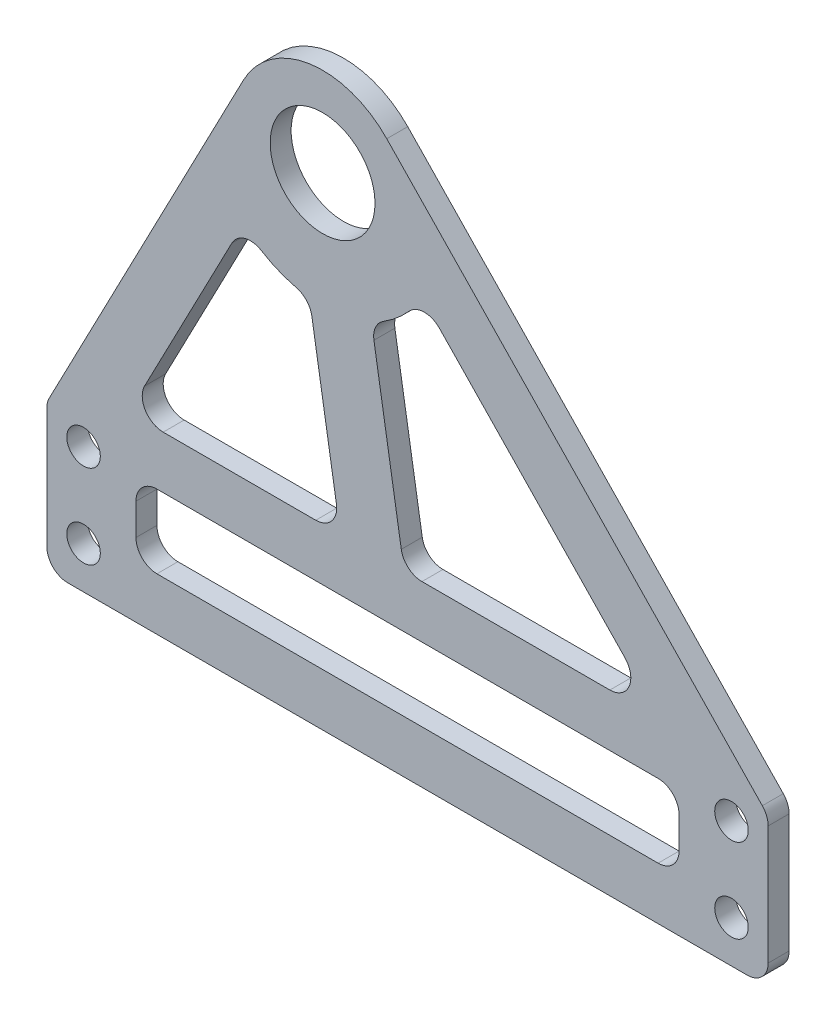
from build123d import *

# Parameters (mm, degrees)
SKETCH_1_R          = 5
SKETCH_1_R_2        = 1.6
EXTRUDE_1_DEPTH     = 2
SKETCH_6_W          = 51.8
SKETCH_6_H          = 7
CUT_EXTRUDE_4_DEPTH = 63.659795723
FILLET_5_R          = 2
FILLET_6_R          = 2


with BuildPart() as part:
    # 草图1 → 凸台-拉伸1 (new body)
    with BuildSketch(Plane.XY):
        with BuildLine():
            Line((-26.3, -32.06084855), (-26.3, -46))
            Line((-26.3, -46), (42.5, -46))
            Line((42.5, -46), (42.5, -31.867732913))
            Line((42.5, -31.867732913), (6.12172987, 5.896984263))
            ThreePointArc((6.12172987, 5.896984263), (-1.211932074, 8.413157591), (-7.537237585, 3.929382851))
            Line((-7.537237585, 3.929382851), (-26.3, -32.06084855))
        make_face()
        Circle(SKETCH_1_R, mode=Mode.SUBTRACT)
        with Locations((-22.8, -34)):
            Circle(SKETCH_1_R_2, mode=Mode.SUBTRACT)
        with Locations((-22.8, -42)):
            Circle(SKETCH_1_R_2, mode=Mode.SUBTRACT)
        with Locations(Location((39, -42, 0), (0, 0, 180))):
            Circle(SKETCH_1_R_2, mode=Mode.SUBTRACT)
        with Locations(Location((39, -34, 0), (0, 0, 180))):
            Circle(SKETCH_1_R_2, mode=Mode.SUBTRACT)
    extrude(amount=EXTRUDE_1_DEPTH)

    # 草图6 → 切除-拉伸4 (cut, through all)
    with BuildSketch(Plane.XY.offset(2)):
        with BuildLine():
            Line((-7.552516715, -7.997467804), (-18.501752281, -29))
            Line((-18.501752281, -29), (1.7, -29))
            Line((1.7, -29), (-1.253662685, -10.928326948))
            ThreePointArc((-1.253662685, -10.928326948), (-4.640547676, -9.973230032), (-7.552516715, -7.997467804))
        make_face()
        with BuildLine():
            Line((4.667768527, -9.960518911), (7.779611281, -29))
            Line((7.779611281, -29), (32.100819179, -29))
            Line((32.100819179, -29), (9.502706469, -5.540629004))
            ThreePointArc((9.502706469, -5.540629004), (7.421889726, -8.118839381), (4.667768527, -9.960518911))
        make_face()
        with Locations((8.1, -37.5)):
            Rectangle(SKETCH_6_W, SKETCH_6_H)
    extrude(amount=-CUT_EXTRUDE_4_DEPTH, mode=Mode.SUBTRACT)

    # 圆角5
    fillet_5_edges = [part.edges().sort_by_distance(p)[0] for p in [
        (-17.8, -41, 1),
        (-17.8, -34, 1),
        (34, -34, 1),
        (34, -41, 1),
        (4.667768527, -9.960518911, 1),
        (9.502706469, -5.540629004, 1),
        (32.100819179, -29, 1),
        (7.779611281, -29, 1),
        (-7.552516715, -7.997467804, 1),
        (-1.253662685, -10.928326948, 1),
        (1.7, -29, 1),
        (-18.501752281, -29, 1),
    ]]
    fillet(fillet_5_edges, radius=FILLET_5_R)

    # 圆角6
    fillet_6_edges = [part.edges().sort_by_distance(p)[0] for p in [
        (42.5, -31.867732913, 1),
        (42.5, -46, 1),
        (-26.3, -46, 1),
        (-26.3, -32.06084855, 1),
    ]]
    fillet(fillet_6_edges, radius=FILLET_6_R)


solid = part.part
